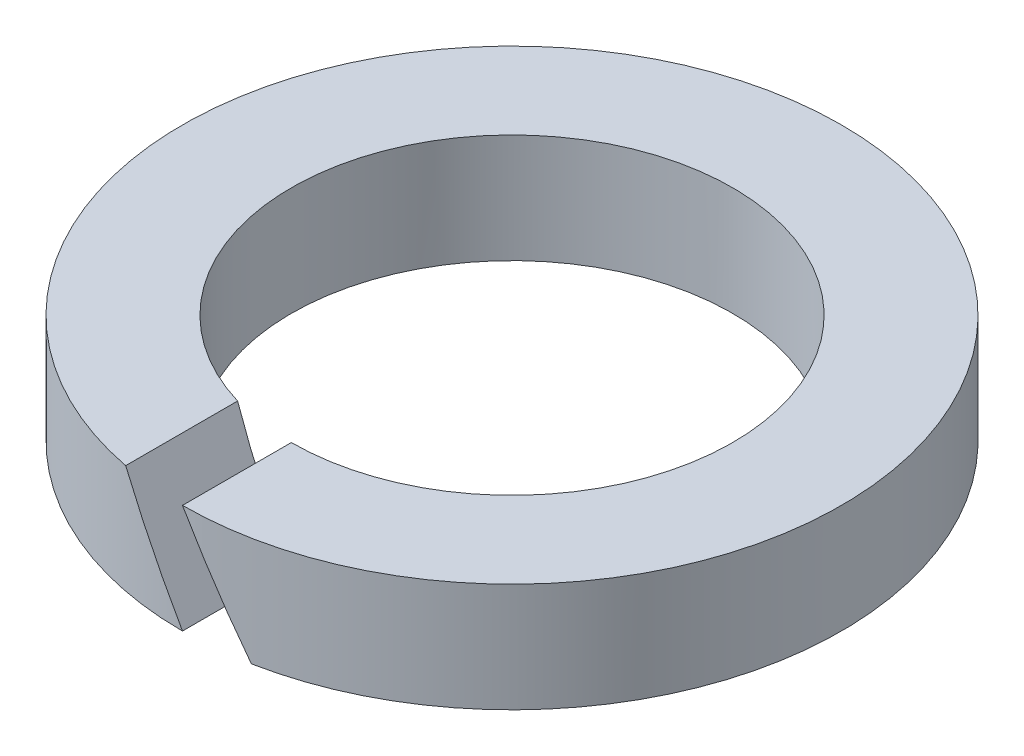
from build123d import *

# Parameters (mm, degrees)
SKETCH1_R           = 27.25
SKETCH1_R_2         = 18.25
BOSS_EXTRUDE1_DEPTH = 4.5
CUT_EXTRUDE1_DEPTH  = 39.799162362


with BuildPart() as part:
    # Sketch1 → Boss-Extrude1 (new, symmetric)
    with BuildSketch(Plane(origin=(0, 0, 0), x_dir=(1, 0, 0), z_dir=(0, 1, 0))):
        with Locations(Location((0, 0, 0), (0, 0, 270))):
            Circle(SKETCH1_R)
        with Locations(Location((0, 0, 0), (0, 0, 270))):
            Circle(SKETCH1_R_2, mode=Mode.SUBTRACT)
    extrude(amount=BOSS_EXTRUDE1_DEPTH, both=True)

    # Sketch2 → Cut-Extrude1 (cut, through all)
    with BuildSketch(Plane.XY):
        Polygon((0, 4.5), (-5.196152423, 4.5), (0, -4.5), (5.196152423, -4.5), align=None)
    extrude(amount=CUT_EXTRUDE1_DEPTH, mode=Mode.SUBTRACT)


solid = part.part
